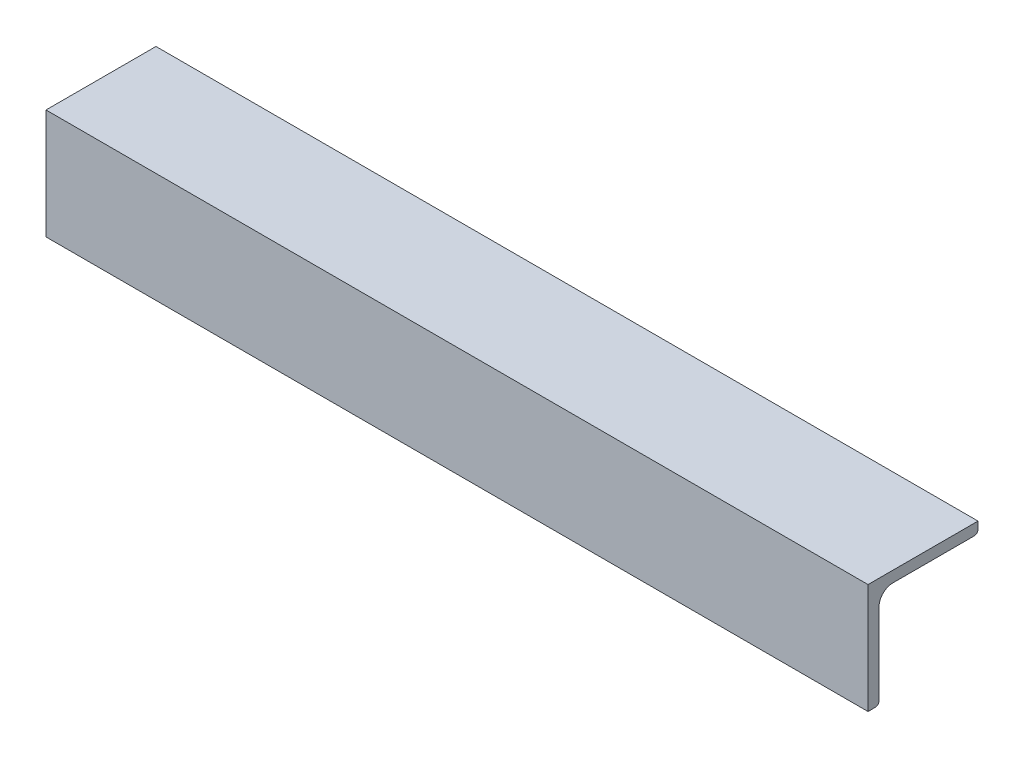
from build123d import *

# Parameters (mm, degrees)
MEMBER_4X4_1_DEPTH = 299


with BuildPart() as part:
    # Sketch13 → Member 4X4_1 (new body)
    with BuildSketch(Plane(origin=(0, 0, 0), x_dir=(0, 0, -1), z_dir=(1, 0, 0))):
        with BuildLine():
            Line((40, 0), (0, 0))
            Line((0, 0), (0, -40))
            Line((0, -40), (2.666666667, -40))
            ThreePointArc((2.666666667, -40), (3.609475708, -39.609475708), (4, -38.666666667))
            Line((4, -38.666666667), (4, -9))
            ThreePointArc((4, -9), (5.464466094, -5.464466094), (9, -4))
            Line((9, -4), (38.666666667, -4))
            ThreePointArc((38.666666667, -4), (39.609475708, -3.609475708), (40, -2.666666667))
            Line((40, -2.666666667), (40, 0))
        make_face()
    extrude(amount=MEMBER_4X4_1_DEPTH)


solid = part.part
